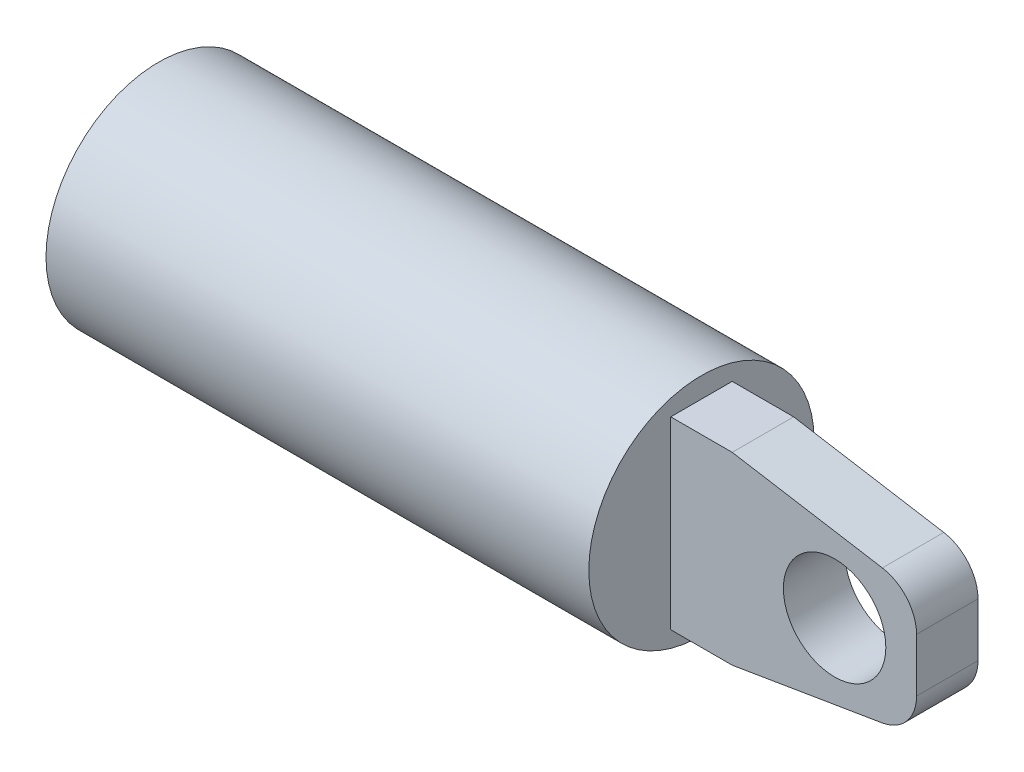
from build123d import *

# Parameters (mm, degrees)
SKETCH1_W                      = 53
SKETCH1_H                      = 11
BOSS_EXTRUDE1_DEPTH            = 6
F_10_0_10_DIAMETER_HOLE1_D     = 10
F_10_0_10_DIAMETER_HOLE1_DEPTH = 14
FILLET1_R                      = 4


with BuildPart() as part:
    # Sketch1 → Revolve1 (revolve)
    with BuildSketch(Plane.XY, mode=Mode.PRIVATE) as revolve1_sk:
        with Locations((26.5, 5.5)):
            Rectangle(SKETCH1_W, SKETCH1_H)
    revolve(revolve1_sk.sketch.rotate(Axis((0, 0, 0), (1, 0, 0)), 270), axis=Axis((0, 0, 0), (1, 0, 0)))

    # Sketch2 → Boss-Extrude1 (add)
    with BuildSketch(Plane.XY.offset(3)):
        Polygon((77, -6), (77, 6), (59, 9), (53, 9), (53, -9), (59, -9), align=None)
    extrude(amount=-BOSS_EXTRUDE1_DEPTH)

    # Ø10.0 (10) Diameter Hole1
    with Locations(Plane(origin=(0, 0, -3), x_dir=(-1, 0, 0), z_dir=(0, 0, -1))):
        with Locations((-69, 0)):
            Hole(F_10_0_10_DIAMETER_HOLE1_D / 2, depth=F_10_0_10_DIAMETER_HOLE1_DEPTH)

    # Sketch5 → CBORE for M13 SHSS1 (revolve, cut)
    with BuildSketch(Plane.ZX):
        Polygon((0, 0), (0, 50), (8, 50), (8, 5), (4, 5), (4, 0), align=None)
    revolve(axis=Axis((-6.35, 0, 0), (1, 0, 0)), mode=Mode.SUBTRACT)

    # Fillet1
    fillet1_edges = [part.edges().sort_by_distance(p)[0] for p in [
        (77, -6, 0),
        (77, 6, 0),
    ]]
    fillet(fillet1_edges, radius=FILLET1_R)


solid = part.part
